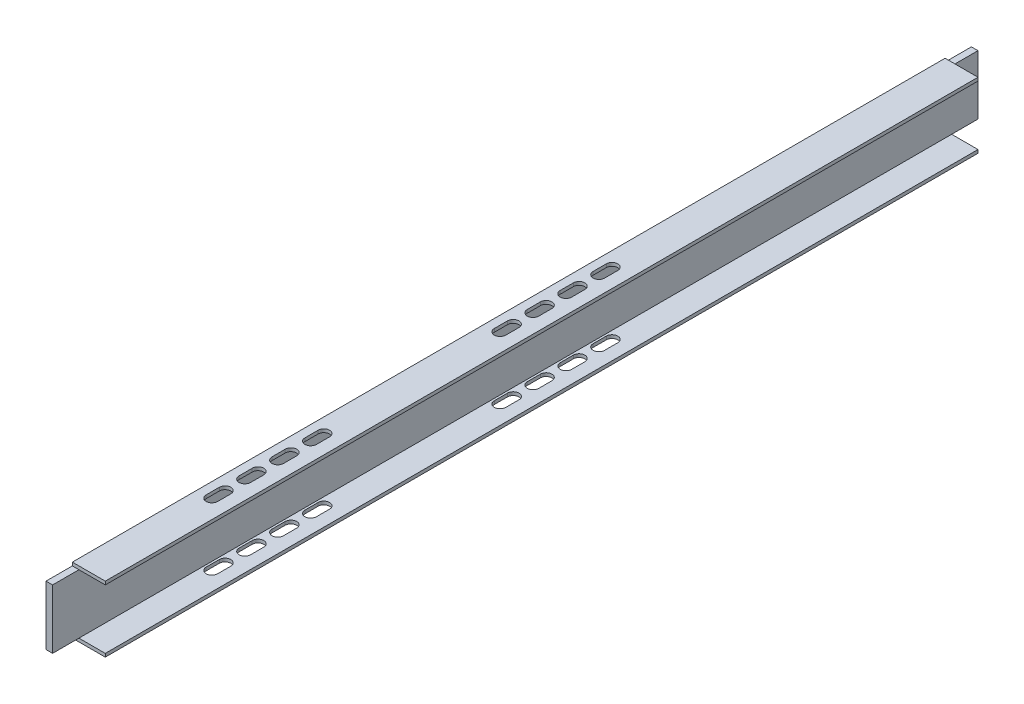
from build123d import *

# Parameters (mm, degrees)
EXTRUDE1_DEPTH         = 1124
SKETCH2_W              = 32
SKETCH2_H              = 32
CUT_EXTRUDE1_DEPTH     = 1128.553102962
SKETCH3_W              = 32
SKETCH3_H              = 4
CUT_EXTRUDE2_DEPTH     = 1200
CUT_EXTRUDE3_DEPTH     = 1128.553102962
LPATTERN1_COUNT        = 4
LPATTERN1_PITCH        = 40
LPATTERN2_COUNT        = 2
LPATTERN2_PITCH        = 350
LPATTERN2_COPY_1_DEPTH = 1128.553102962
LPATTERN2_COPY_2_DEPTH = 1128.553102962
LPATTERN2_COPY_3_DEPTH = 1128.553102962


with BuildPart() as part:
    # Sketch1 → Extrude1 (new body)
    with BuildSketch(Plane.XY):
        Polygon((0, 0), (-40, 0), (-40, 80), (0, 80), (0, 76), (-32, 76), (-32, 4), (0, 4), align=None)
    extrude(amount=EXTRUDE1_DEPTH)

    # Sketch2 → Cut-Extrude1 (cut, through all)
    with BuildSketch(Plane(origin=(0, 80, 0), x_dir=(1, 0, 0), z_dir=(0, 1, 0))):
        with Locations((-16, -16)):
            Rectangle(SKETCH2_W, SKETCH2_H)
        with Locations((-16, -1108)):
            Rectangle(SKETCH2_W, SKETCH2_H)
    extrude(amount=-CUT_EXTRUDE1_DEPTH, mode=Mode.SUBTRACT)

    # Sketch3 → Cut-Extrude2 (cut)
    with BuildSketch(Plane(origin=(-32, 0, 0), x_dir=(0, 0, -1), z_dir=(1, 0, 0))):
        with Locations((-1108, 78)):
            Rectangle(SKETCH3_W, SKETCH3_H)
        with Locations((-1108, 2)):
            Rectangle(SKETCH3_W, SKETCH3_H)
        with Locations((-16, 78)):
            Rectangle(SKETCH3_W, SKETCH3_H)
        with Locations((-16, 2)):
            Rectangle(SKETCH3_W, SKETCH3_H)
    extrude(amount=-CUT_EXTRUDE2_DEPTH, mode=Mode.SUBTRACT)

    # Sketch4 → Cut-Extrude3 (cut, through all)
    with BuildSketch(Plane(origin=(0, 80, 0), x_dir=(1, 0, 0), z_dir=(0, 1, 0))):
        with BuildLine():
            Line((-29.5, -924), (-29.5, -940))
            ThreePointArc((-29.5, -940), (-22.5, -947), (-15.5, -940))
            Line((-15.5, -940), (-15.5, -924))
            ThreePointArc((-15.5, -924), (-22.5, -917), (-29.5, -924))
        make_face()
    cut_extrude3 = extrude(amount=-CUT_EXTRUDE3_DEPTH, mode=Mode.SUBTRACT)

    # LPattern1: Cut-Extrude3 ×4
    with Locations(*[(0, 0, -i * LPATTERN1_PITCH) for i in range(1, LPATTERN1_COUNT)]):
        add(cut_extrude3, mode=Mode.SUBTRACT)

    # LPattern2: Cut-Extrude3 ×2
    with Locations(*[(0, 0, -i * LPATTERN2_PITCH) for i in range(1, LPATTERN2_COUNT)]):
        add(cut_extrude3, mode=Mode.SUBTRACT)

    # LPattern2 copy 1 sketch → LPattern2 copy 1 (cut, through all)
    with BuildSketch(Plane(origin=(0, 80, -390), x_dir=(1, 0, 0), z_dir=(0, 1, 0))):
        with BuildLine():
            Line((-29.5, -924), (-29.5, -940))
            ThreePointArc((-29.5, -940), (-22.5, -947), (-15.5, -940))
            Line((-15.5, -940), (-15.5, -924))
            ThreePointArc((-15.5, -924), (-22.5, -917), (-29.5, -924))
        make_face()
    extrude(amount=-LPATTERN2_COPY_1_DEPTH, mode=Mode.SUBTRACT)

    # LPattern2 copy 2 sketch → LPattern2 copy 2 (cut, through all)
    with BuildSketch(Plane(origin=(0, 80, -430), x_dir=(1, 0, 0), z_dir=(0, 1, 0))):
        with BuildLine():
            Line((-29.5, -924), (-29.5, -940))
            ThreePointArc((-29.5, -940), (-22.5, -947), (-15.5, -940))
            Line((-15.5, -940), (-15.5, -924))
            ThreePointArc((-15.5, -924), (-22.5, -917), (-29.5, -924))
        make_face()
    extrude(amount=-LPATTERN2_COPY_2_DEPTH, mode=Mode.SUBTRACT)

    # LPattern2 copy 3 sketch → LPattern2 copy 3 (cut, through all)
    with BuildSketch(Plane(origin=(0, 80, -470), x_dir=(1, 0, 0), z_dir=(0, 1, 0))):
        with BuildLine():
            Line((-29.5, -924), (-29.5, -940))
            ThreePointArc((-29.5, -940), (-22.5, -947), (-15.5, -940))
            Line((-15.5, -940), (-15.5, -924))
            ThreePointArc((-15.5, -924), (-22.5, -917), (-29.5, -924))
        make_face()
    extrude(amount=-LPATTERN2_COPY_3_DEPTH, mode=Mode.SUBTRACT)


solid = part.part
